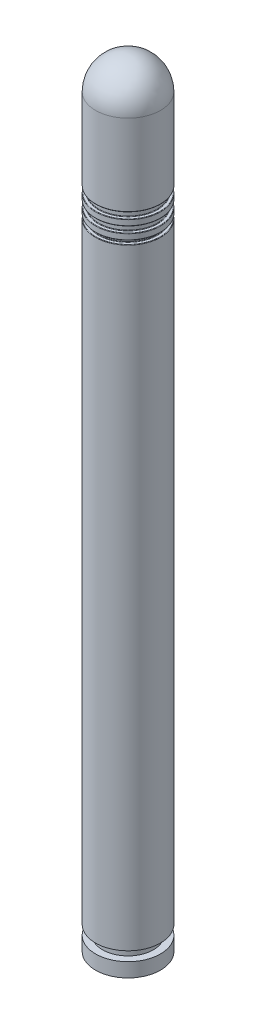
from build123d import *


with BuildPart() as part:
    # Sketch1 → Revolve1 (revolve)
    with BuildSketch(Plane.XY, mode=Mode.PRIVATE) as revolve1_sk:
        with BuildLine():
            Line((2, 0.2), (3.45, 0.2))
            Line((3.45, 0.2), (3.45, 1.7))
            Line((3.45, 1.7), (2.7, 1.7))
            Line((2.7, 1.7), (2.7, 2.7))
            Line((2.7, 2.7), (3.45, 2.7))
            Line((3.45, 2.7), (3.45, 67.65))
            ThreePointArc((3.45, 67.65), (3.435355339, 67.685355339), (3.4, 67.7))
            Line((3.4, 67.7), (3.15, 67.7))
            ThreePointArc((3.15, 67.7), (3.114644661, 67.714644661), (3.1, 67.75))
            Line((3.1, 67.75), (3.1, 68.05))
            ThreePointArc((3.1, 68.05), (3.114644661, 68.085355339), (3.15, 68.1))
            Line((3.15, 68.1), (3.4, 68.1))
            ThreePointArc((3.4, 68.1), (3.435355339, 68.114644661), (3.45, 68.15))
            Line((3.45, 68.15), (3.45, 68.7))
            ThreePointArc((3.45, 68.7), (3.435355339, 68.735355339), (3.4, 68.75))
            Line((3.4, 68.75), (3.15, 68.75))
            ThreePointArc((3.15, 68.75), (3.114644661, 68.764644661), (3.1, 68.8))
            Line((3.1, 68.8), (3.1, 69.35))
            ThreePointArc((3.1, 69.35), (3.114644661, 69.385355339), (3.15, 69.4))
            Line((3.15, 69.4), (3.4, 69.4))
            ThreePointArc((3.4, 69.4), (3.435355339, 69.414644661), (3.45, 69.45))
            Line((3.45, 69.45), (3.45, 70))
            ThreePointArc((3.45, 70), (3.435355339, 70.035355339), (3.4, 70.05))
            Line((3.4, 70.05), (3.15, 70.05))
            ThreePointArc((3.15, 70.05), (3.114644661, 70.064644661), (3.1, 70.1))
            Line((3.1, 70.1), (3.1, 70.65))
            ThreePointArc((3.1, 70.65), (3.114644661, 70.685355339), (3.15, 70.7))
            Line((3.15, 70.7), (3.4, 70.7))
            ThreePointArc((3.4, 70.7), (3.435355339, 70.714644661), (3.45, 70.75))
            Line((3.45, 70.75), (3.45, 79.35))
            ThreePointArc((3.45, 79.35), (2.439518395, 81.789518395), (0, 82.8))
            Line((0, 82.8), (0, 79.35))
            Line((0, 79.35), (2, 79.35))
            Line((2, 79.35), (2, 0.2))
        make_face()
    revolve(revolve1_sk.sketch.rotate(Axis((0, -7.873710816, 0), (0, 1, 0)), 90), axis=Axis((0, -7.873710816, 0), (0, 1, 0)))


solid = part.part
